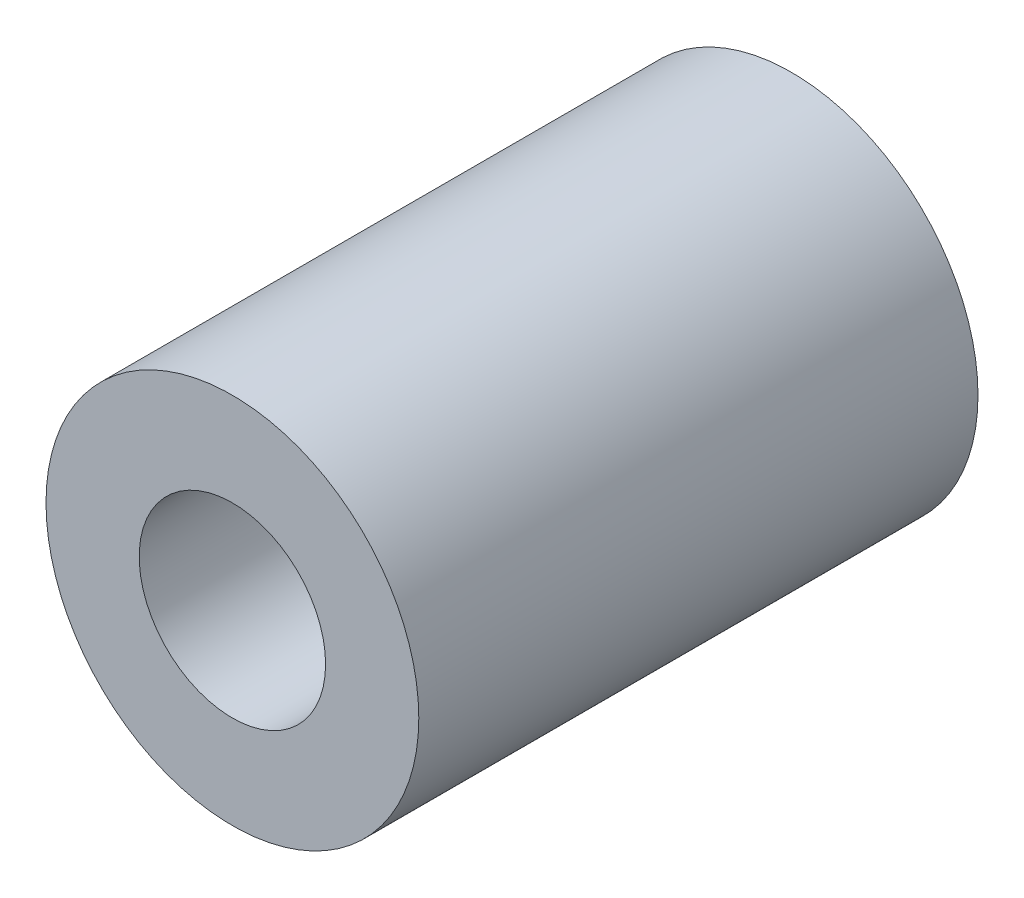
SolidWorks part; units mm, degrees
ref_plane "前视基准面" through (0, 0, 0) normal (0, 0, 1) x (1, 0, 0)
ref_plane "上视基准面" through (0, 0, 0) normal (0, 1, 0) x (1, 0, 0)
ref_plane "右视基准面" through (0, 0, 0) normal (1, 0, 0) x (0, 0, -1)
sketch "草图1" plane through (0, 0, 0) normal (0, 0, 1) x (1, 0, 0)
  circle A0 centre (0, 0) radius 10
  dimension "D1" = 20
extrude "凸台-拉伸1" add sketch "草图1" along normal mid plane 30
hole_wizard "打孔尺寸(%根据)内六角圆柱头螺钉的类型1" positions "3D草图1" profile "草图2" counterbore size "M5" standard "GB" end condition up to next
sketch3d "3D草图1"
  circle A0 centre (0, 0, 15) radius 10 construction
  point P0 (0, 0, 15)
  point P5 (0, 0, 25)
sketch "草图2" plane through (0, 0, 15) normal (1, 0, 0) x (0, -1, 0)
  line L0 (0, 0) -> (0, 30)
  line L1 (0, 30) -> (2.75, 30)
  line L3 (2.75, 30) -> (2.75, 12)
  line L4 (2.75, 12) -> (5, 12)
  line L5 (5, 12) -> (5, 0)
  line L7 (5, 0) -> (0, 0)
  line L11 (0, -6.35) -> (0, 107.95) construction
  dimension "通孔孔直径" = 5.5
  dimension "通孔孔深度" = 30
  dimension "柱形沉头孔直径" = 10
  dimension "柱形沉头孔深度" = 12
